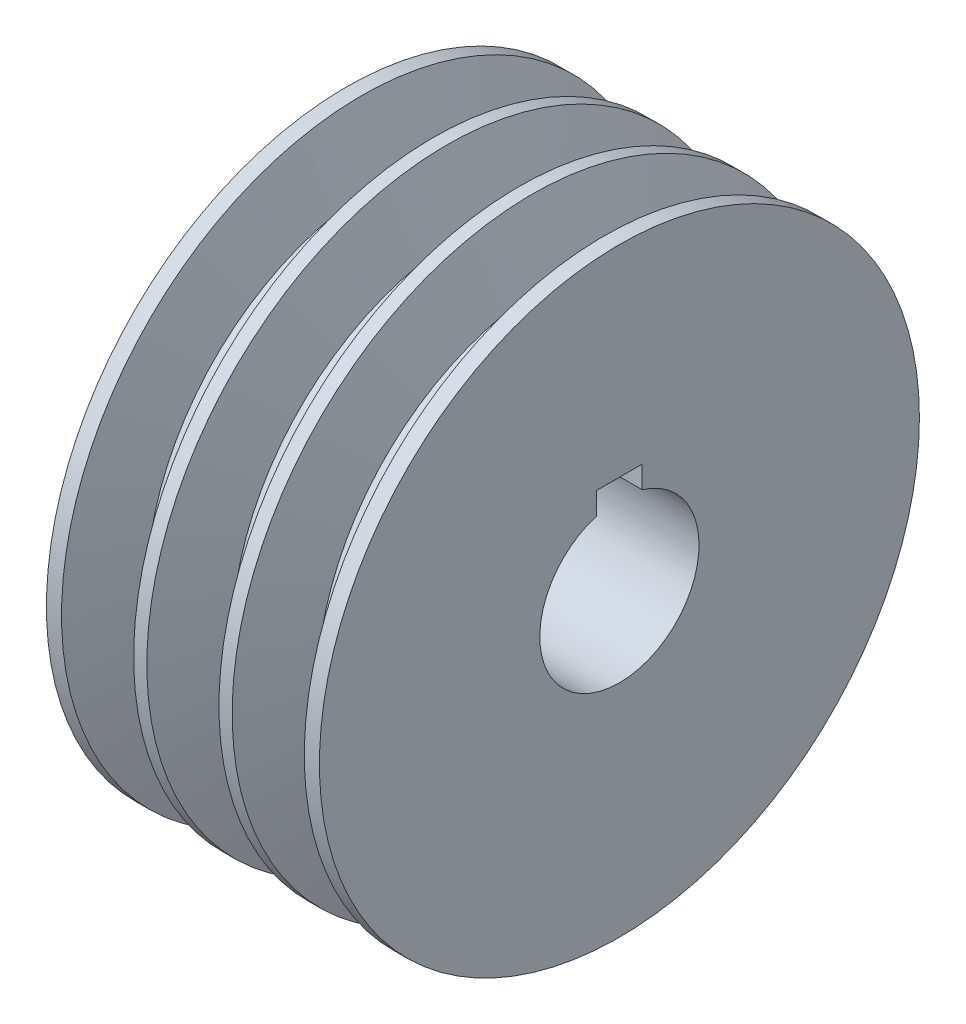
from build123d import *

# Parameters (mm, degrees)
SKETCH8_R           = 25
SKETCH8_R_2         = 14
BOSS_EXTRUDE2_DEPTH = 4
CUT_EXTRUDE5_REACH  = 92.935
SKETCH9_W           = 8
SKETCH9_H           = 6.6


with BuildPart() as part:
    # Sketch1 → Revolve1 (revolve)
    with BuildSketch(Plane.XY, mode=Mode.PRIVATE) as revolve1_sk:
        Polygon((6.158767395, 41.3), (2.658151092, 52.75), (0, 52.75), (0, 14), (48, 14), (48, 52.75), (45.341848908, 52.75), (41.841232605, 41.3), (36.161232605, 41.3), (32.660616303, 52.75), (30.340616303, 52.75), (26.84, 41.3), (21.16, 41.3), (17.659383697, 52.75), (15.339383697, 52.75), (11.838767395, 41.3), align=None)
    revolve(revolve1_sk.sketch.rotate(Axis((0, 0, 0), (1, 0, 0)), 270), axis=Axis((0, 0, 0), (1, 0, 0)))

    # Sketch8 → Boss-Extrude2 (add)
    with BuildSketch(Plane.ZY):
        Circle(SKETCH8_R)
        with Locations(Location((0, 0, 0), (0, 0, 180))):
            Circle(SKETCH8_R_2, mode=Mode.SUBTRACT)
    extrude(amount=BOSS_EXTRUDE2_DEPTH)

    # Sketch9 → Cut-Extrude5 (cut, up to next)
    with BuildSketch(Plane.ZY.offset(4), mode=Mode.PRIVATE) as cut_extrude5_sk1:
        with Locations((0, 14)):
            Rectangle(SKETCH9_W, SKETCH9_H)
    cut_extrude5_tool1 = extrude(cut_extrude5_sk1.sketch, amount=-CUT_EXTRUDE5_REACH, mode=Mode.PRIVATE) & part.part
    add(cut_extrude5_tool1.solids().sort_by_distance((-4, 14, 0))[0], mode=Mode.SUBTRACT)


solid = part.part
